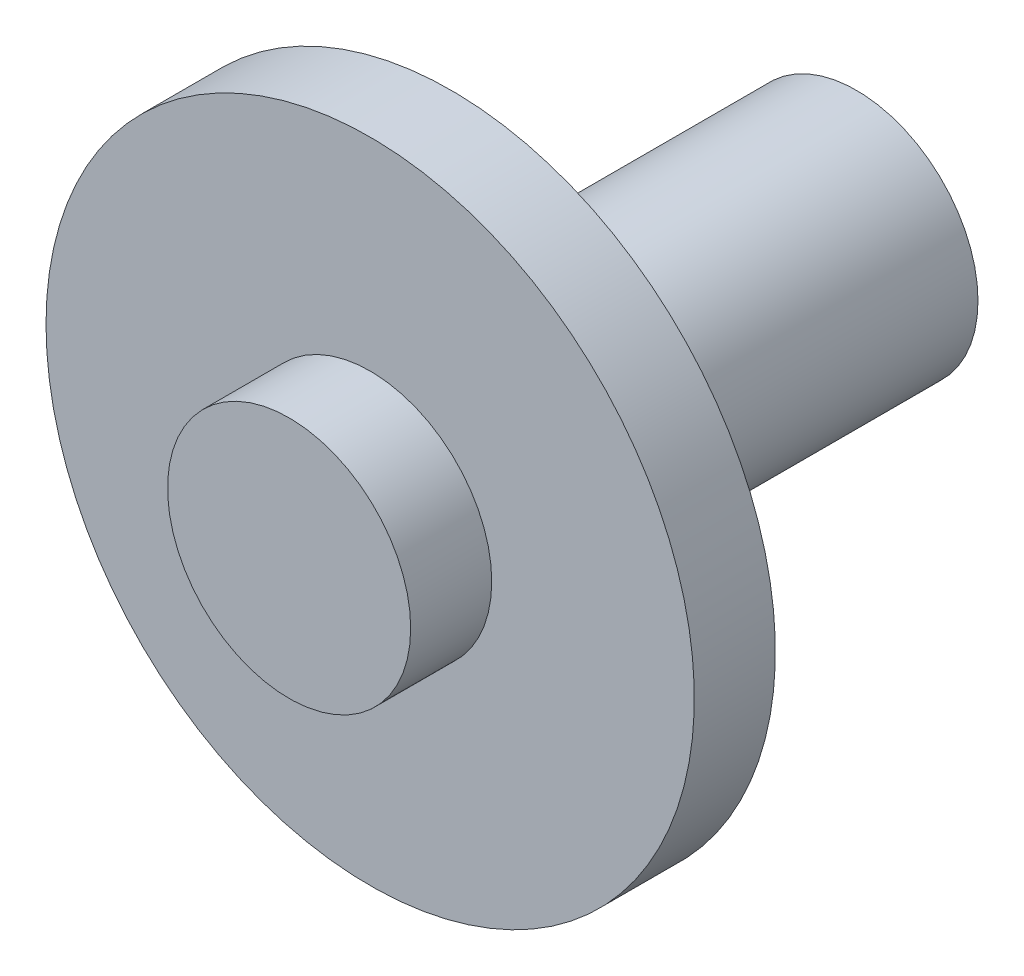
SolidWorks part; units mm, degrees
ref_plane "Front plane" through (0, 0, 0) normal (0, 0, 1) x (1, 0, 0)
ref_plane "Top plane" through (0, 0, 0) normal (0, 1, 0) x (1, 0, 0)
ref_plane "Right plane" through (0, 0, 0) normal (1, 0, 0) x (0, 0, -1)
sketch "Sketch 1" plane through (0, 0, 0) normal (0, 0, 1) x (1, 0, 0)
  circle A0 centre (0, 0) radius 1.5
  dimension "D1" = 3
extrude "Boss-Extrude 1" add sketch "Sketch 1" along normal blind 1
sketch "Sketch 2" plane through (0, 0, 0) normal (0, 0, -1) x (-1, 0, 0)
  circle A0 centre (0, 0) radius 4
  dimension "D1" = 8
extrude "Boss-Extrude 2" add sketch "Sketch 2" along normal blind 1
sketch "Sketch 3" plane through (0, 0, -1) normal (0, 0, -1) x (-1, 0, 0)
  circle A0 centre (0, 0) radius 2.5
  dimension "D1" = 5
extrude "Boss-Extrude 3" add sketch "Sketch 3" along normal blind 1
sketch "Sketch 4" plane through (0, 0, -2) normal (0, 0, -1) x (-1, 0, 0)
  circle A0 centre (0, 0) radius 1.5
  dimension "D1" = 3
extrude "Boss-Extrude 4" add sketch "Sketch 4" along normal blind 4
sketch "Sketch 5" plane through (0, 0, 0) normal (0, 1, 0) x (1, 0, 0)
  line L2 (1.5, 2.0031) -> (2.5, 2)
  line L4 (2.5, 2) -> (2.5, 1)
  line L6 (0, 2.0031) -> (0, 4.8142) construction
  arc A0 (1.5, 2.0031) -> (2.5, 1) centre (2.5, 2) ccw
revolve "Cut-Revolve 2" cut sketch "Sketch 5" angle 360 about L6
